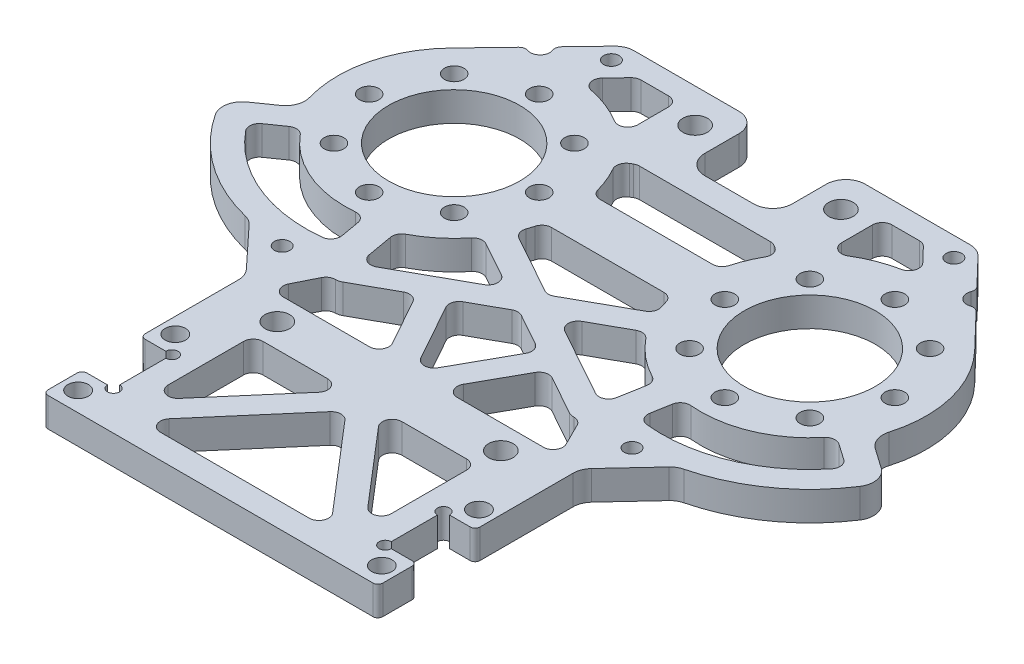
from build123d import *

# Parameters (mm, degrees)
SKETCH_1_R              = 13.5
SKETCH_1_R_2            = 2.525
SKETCH_1_R_3            = 2.01
SKETCH_1_R_4            = 2.1
SKETCH_1_R_5            = 1.6
EXTRUDE_1_DEPTH         = 6
CUT_EXTRUDE_1_DEPTH     = 111.547291087
FILLET_R2_R             = 2
FILLET_R1_R             = 1
FILLET_R4_R             = 4
CUT_EXTRUDE_73_20_DEPTH = 110.7530004


with BuildPart() as part:
    # 草图1 → 凸台-拉伸1 (new body)
    with BuildSketch(Plane(origin=(0, 0, 0), x_dir=(1, 0, 0), z_dir=(0, 1, 0))):
        with BuildLine():
            Line((-36.261062267, 35), (-9, 35))
            Line((-9, 35), (-9, 20))
            Line((-9, 20), (9, 20))
            Line((9, 20), (9, 35))
            Line((9, 35), (36.261062267, 35))
            Line((36.261062267, 35), (53.909452324, 16.624766472))
            ThreePointArc((53.909452324, 16.624766472), (60.203109588, 4.346632924), (58.696156922, -9.368022698))
            Line((58.696156922, -9.368022698), (68.25790113, -16.063228071))
            ThreePointArc((68.25790113, -16.063228071), (58.255238391, -28.130066659), (44.031297301, -34.713481825))
            Line((44.031297301, -34.713481825), (34.45, -45))
            Line((34.45, -45), (34.45, -66.75))
            Line((34.45, -66.75), (29.2, -66.75))
            ThreePointArc((29.2, -66.75), (27.066116524, -65.866116524), (27.95, -68))
            Line((27.95, -68), (27.95, -77.5))
            ThreePointArc((27.95, -77.5), (27.066116524, -79.633883476), (29.2, -78.75))
            Line((29.2, -78.75), (34.45, -78.75))
            Line((34.45, -78.75), (34.45, -86.75))
            Line((34.45, -86.75), (-34.45, -86.75))
            Line((-34.45, -86.75), (-34.45, -78.75))
            Line((-34.45, -78.75), (-29.2, -78.75))
            ThreePointArc((-29.2, -78.75), (-27.066116524, -79.633883476), (-27.95, -77.5))
            Line((-27.95, -77.5), (-27.95, -68))
            ThreePointArc((-27.95, -68), (-27.066116524, -65.866116524), (-29.2, -66.75))
            Line((-29.2, -66.75), (-34.45, -66.75))
            Line((-34.45, -66.75), (-34.45, -45))
            Line((-34.45, -45), (-44.031297301, -34.713481825))
            ThreePointArc((-44.031297301, -34.713481825), (-58.255238391, -28.130066659), (-68.25790113, -16.063228071))
            Line((-68.25790113, -16.063228071), (-58.696156922, -9.368022698))
            ThreePointArc((-58.696156922, -9.368022698), (-60.203109588, 4.346632924), (-53.909452324, 16.624766472))
            Line((-53.909452324, 16.624766472), (-36.261062267, 35))
        make_face()
        with Locations(Location((-36.6, 0, 0), (0, 0, 270))):
            Circle(SKETCH_1_R, mode=Mode.SUBTRACT)
        with Locations(Location((-15, 28, 0), (0, 0, 270))):
            Circle(SKETCH_1_R_2, mode=Mode.SUBTRACT)
        with Locations(Location((15, 28, 0), (0, 0, 270))):
            Circle(SKETCH_1_R_2, mode=Mode.SUBTRACT)
        with Locations(Location((-23, -50, 0), (0, 0, 270))):
            Circle(SKETCH_1_R_2, mode=Mode.SUBTRACT)
        with Locations(Location((23, -50, 0), (0, 0, 270))):
            Circle(SKETCH_1_R_2, mode=Mode.SUBTRACT)
        with Locations(Location((36.6, 0, 0), (0, 0, 90))):
            Circle(SKETCH_1_R, mode=Mode.SUBTRACT)
        with Locations(Location((-36.6, 17.5, 0), (0, 0, 270))):
            Circle(SKETCH_1_R_3, mode=Mode.SUBTRACT)
        with Locations(Location((-24.225631329, 12.374368671, 0), (0, 0, 270))):
            Circle(SKETCH_1_R_3, mode=Mode.SUBTRACT)
        with Locations(Location((-19.1, 0, 0), (0, 0, 270))):
            Circle(SKETCH_1_R_3, mode=Mode.SUBTRACT)
        with Locations(Location((-24.225631329, -12.374368671, 0), (0, 0, 270))):
            Circle(SKETCH_1_R_3, mode=Mode.SUBTRACT)
        with Locations(Location((-36.6, -17.5, 0), (0, 0, 270))):
            Circle(SKETCH_1_R_3, mode=Mode.SUBTRACT)
        with Locations(Location((-48.974368671, -12.374368671, 0), (0, 0, 270))):
            Circle(SKETCH_1_R_3, mode=Mode.SUBTRACT)
        with Locations(Location((-54.1, 0, 0), (0, 0, 270))):
            Circle(SKETCH_1_R_3, mode=Mode.SUBTRACT)
        with Locations(Location((-48.974368671, 12.374368671, 0), (0, 0, 270))):
            Circle(SKETCH_1_R_3, mode=Mode.SUBTRACT)
        with Locations(Location((48.974368671, 12.374368671, 0), (0, 0, 90))):
            Circle(SKETCH_1_R_3, mode=Mode.SUBTRACT)
        with Locations(Location((54.1, 0, 0), (0, 0, 90))):
            Circle(SKETCH_1_R_3, mode=Mode.SUBTRACT)
        with Locations(Location((48.974368671, -12.374368671, 0), (0, 0, 90))):
            Circle(SKETCH_1_R_3, mode=Mode.SUBTRACT)
        with Locations(Location((36.6, -17.5, 0), (0, 0, 90))):
            Circle(SKETCH_1_R_3, mode=Mode.SUBTRACT)
        with Locations(Location((24.225631329, -12.374368671, 0), (0, 0, 90))):
            Circle(SKETCH_1_R_3, mode=Mode.SUBTRACT)
        with Locations(Location((19.1, 0, 0), (0, 0, 90))):
            Circle(SKETCH_1_R_3, mode=Mode.SUBTRACT)
        with Locations(Location((24.225631329, 12.374368671, 0), (0, 0, 90))):
            Circle(SKETCH_1_R_3, mode=Mode.SUBTRACT)
        with Locations(Location((36.6, 17.5, 0), (0, 0, 90))):
            Circle(SKETCH_1_R_3, mode=Mode.SUBTRACT)
        with Locations(Location((-31.25, -82.75, 0), (0, 0, 270))):
            Circle(SKETCH_1_R_4, mode=Mode.SUBTRACT)
        with Locations(Location((-31.25, -62.75, 0), (0, 0, 270))):
            Circle(SKETCH_1_R_4, mode=Mode.SUBTRACT)
        with Locations(Location((31.25, -82.75, 0), (0, 0, 90))):
            Circle(SKETCH_1_R_4, mode=Mode.SUBTRACT)
        with Locations(Location((31.25, -62.75, 0), (0, 0, 90))):
            Circle(SKETCH_1_R_4, mode=Mode.SUBTRACT)
        with Locations(Location((-35.25, 31, 0), (0, 0, 270))):
            Circle(SKETCH_1_R_5, mode=Mode.SUBTRACT)
        with Locations(Location((35.25, 31, 0), (0, 0, 90))):
            Circle(SKETCH_1_R_5, mode=Mode.SUBTRACT)
        with Locations(Location((-36, -36, 0), (0, 0, 270))):
            Circle(SKETCH_1_R_5, mode=Mode.SUBTRACT)
        with Locations(Location((36, -36, 0), (0, 0, 90))):
            Circle(SKETCH_1_R_5, mode=Mode.SUBTRACT)
        with BuildLine():
            Line((-55.030920997, -12.905469818), (-61.584137351, -17.494081309))
            ThreePointArc((-61.584137351, -17.494081309), (-48.271844687, -28.178325742), (-31.303730581, -30.036636467))
            Line((-31.303730581, -30.036636467), (-32.692916002, -22.158174443))
            ThreePointArc((-32.692916002, -22.158174443), (-45.210377228, -20.787289482), (-55.030920997, -12.905469818))
        make_face(mode=Mode.SUBTRACT)
        with BuildLine():
            Line((55.030920997, -12.905469818), (61.584137351, -17.494081309))
            ThreePointArc((61.584137351, -17.494081309), (48.271844687, -28.178325742), (31.303730581, -30.036636467))
            Line((31.303730581, -30.036636467), (32.692916002, -22.158174443))
            ThreePointArc((32.692916002, -22.158174443), (45.210377228, -20.787289482), (55.030920997, -12.905469818))
        make_face(mode=Mode.SUBTRACT)
    extrude(amount=EXTRUDE_1_DEPTH)

    # 草图3 → 切除-拉伸1 (cut, through all)
    with BuildSketch(Plane(origin=(0, 6, 0), x_dir=(1, 0, 0), z_dir=(0, 1, 0))):
        with BuildLine():
            Line((-35.748265569, 23.984881664), (-29.490856678, 30.5))
            Line((-29.490856678, 30.5), (-21, 30.5))
            Line((-21, 30.5), (-21, 18.238420984))
            ThreePointArc((-21, 18.238420984), (-27.886771893, 22.362460866), (-35.748265569, 23.984881664))
        make_face()
        with BuildLine():
            ThreePointArc((35.748265569, 23.984881664), (27.886771893, 22.362460866), (21, 18.238420984))
            Line((21, 18.238420984), (21, 30.5))
            Line((21, 30.5), (29.490856678, 30.5))
            Line((29.490856678, 30.5), (35.748265569, 23.984881664))
        make_face()
        with BuildLine():
            Line((-13.126610811, 5), (13.126610811, 5))
            ThreePointArc((13.126610811, 5), (14.513085915, 9.389793725), (16.712198489, 13.434111472))
            Line((16.712198489, 13.434111472), (14, 15))
            Line((14, 15), (-14, 15))
            Line((-14, 15), (-16.712198489, 13.434111472))
            ThreePointArc((-16.712198489, 13.434111472), (-14.513085915, 9.389793725), (-13.126610811, 5))
        make_face()
        with BuildLine():
            Line((13.126610811, -5), (-13.126610811, -5))
            ThreePointArc((-13.126610811, -5), (-13.719828244, -7.245532444), (-14.527321777, -9.423209435))
            ThreePointArc((-14.527321777, -9.423209435), (-14.469211894, -9.452626985), (-14.411888075, -9.483548344))
            Line((-14.411888075, -9.483548344), (0, -17.501639796))
            Line((0, -17.501639796), (14.411888075, -9.483548344))
            ThreePointArc((14.411888075, -9.483548344), (14.469211894, -9.452626985), (14.527321777, -9.423209435))
            ThreePointArc((14.527321777, -9.423209435), (13.719828244, -7.245532444), (13.126610811, -5))
        make_face()
        with BuildLine():
            ThreePointArc((-16.842763472, -13.852855474), (-16.899262321, -13.820451295), (-16.95489785, -13.786586289))
            ThreePointArc((-16.95489785, -13.786586289), (-21.266831345, -18.463313327), (-26.655934481, -21.842975094))
            Line((-26.655934481, -21.842975094), (-24.97170536, -31.394713087))
            Line((-24.97170536, -31.394713087), (-13.806916689, -25.183153842))
            Line((-13.806916689, -25.183153842), (-5.142180472, -20.362505289))
            Line((-5.142180472, -20.362505289), (-16.842763472, -13.852855474))
        make_face()
        with BuildLine():
            ThreePointArc((-23.296885286, -36.184653565), (-24.456132251, -36.499368441), (-25.628351624, -36.237069529))
            Line((-25.628351624, -36.237069529), (-30, -45))
            Line((-30, -45), (-5.642628511, -45))
            Line((-5.642628511, -45), (-13.560695072, -30.767898791))
            Line((-13.560695072, -30.767898791), (-23.296885286, -36.184653565))
        make_face()
        Polygon((9.191387942, -28.337023394), (0, -23.223370782), (-9.191387942, -28.337023394), (0, -44.857819528), align=None)
        with BuildLine():
            ThreePointArc((26.655934481, -21.842975094), (21.266831345, -18.463313327), (16.95489785, -13.786586289))
            ThreePointArc((16.95489785, -13.786586289), (16.899262321, -13.820451295), (16.842763472, -13.852855474))
            Line((16.842763472, -13.852855474), (5.142180472, -20.362505289))
            Line((5.142180472, -20.362505289), (13.806916944, -25.183153984))
            Line((13.806916944, -25.183153984), (24.97170536, -31.394713087))
            Line((24.97170536, -31.394713087), (26.655934481, -21.842975094))
        make_face()
        with BuildLine():
            Line((30, -45), (25.628351624, -36.237069529))
            ThreePointArc((25.628351624, -36.237069529), (24.456132251, -36.499368441), (23.296885286, -36.184653565))
            Line((23.296885286, -36.184653565), (13.560695072, -30.767898791))
            Line((13.560695072, -30.767898791), (5.642628511, -45))
            Line((5.642628511, -45), (30, -45))
        make_face()
        Polygon((-3.29399812, -55), (-22.95, -77.910590426), (-22.95, -55), align=None)
        Polygon((0, -58.839409574), (19.65600188, -81.75), (-19.65600188, -81.75), align=None)
        Polygon((22.95, -55), (3.29399812, -55), (22.95, -77.910590426), align=None)
    extrude(amount=-CUT_EXTRUDE_1_DEPTH, mode=Mode.SUBTRACT)

    # R2 镂空圆角
    fillet_r2_edges = [part.edges().sort_by_distance(p)[0] for p in [
        (-13.126610811, 3, 5),
        (13.126610811, 3, 5),
        (26.655934481, 3, 21.842975094),
        (-26.655934481, 3, 21.842975094),
        (22.95, 3, 55),
        (22.95, 3, 77.910590426),
        (3.29399812, 3, 55),
        (19.65600188, 3, 81.75),
        (-19.65600188, 3, 81.75),
        (0, 3, 58.839409574),
        (-3.29399812, 3, 55),
        (-22.95, 3, 77.910590426),
        (-22.95, 3, 55),
        (-16.712198489, 3, -13.434111472),
        (14, 3, -15),
        (16.712198489, 3, -13.434111472),
        (13.126610811, 3, -5),
        (-13.126610811, 3, -5),
        (-14, 3, -15),
        (21, 3, -30.5),
        (29.490856678, 3, -30.5),
        (35.748265569, 3, -23.984881664),
        (21, 3, -18.238420984),
        (-5.142180472, 3, 20.362505289),
        (-24.97170536, 3, 31.394713087),
        (-16.95489785, 3, 13.786586289),
        (-14.527321777, 3, 9.423209435),
        (14.527321777, 3, 9.423209435),
        (16.95489785, 3, 13.786586289),
        (0, 3, 17.501639796),
        (24.97170536, 3, 31.394713087),
        (5.142180472, 3, 20.362505289),
        (5.642628511, 3, 45),
        (13.560695072, 3, 30.767898791),
        (25.628351624, 3, 36.237069529),
        (30, 3, 45),
        (-13.560695072, 3, 30.767898791),
        (-5.642628511, 3, 45),
        (-30, 3, 45),
        (-25.628351624, 3, 36.237069529),
        (0, 3, 23.223370782),
        (9.191387942, 3, 28.337023394),
        (0, 3, 44.857819528),
        (-9.191387942, 3, 28.337023394),
        (-21, 3, -30.5),
        (-21, 3, -18.238420984),
        (-35.748265569, 3, -23.984881664),
        (61.584137351, 3, 17.494081309),
        (31.303730581, 3, 30.036636467),
        (32.692916002, 3, 22.158174443),
        (55.030920997, 3, 12.905469818),
        (-31.303730581, 3, 30.036636467),
        (-61.584137351, 3, 17.494081309),
        (-55.030920997, 3, 12.905469818),
        (-32.692916002, 3, 22.158174443),
        (-29.490856678, 3, -30.5),
    ]]
    fillet(fillet_r2_edges, radius=FILLET_R2_R)

    # R1 插接圆角
    fillet_r1_edges = [part.edges().sort_by_distance(p)[0] for p in [
        (34.45, 3, 86.75),
        (-34.45, 3, 86.75),
        (-34.45, 3, 78.75),
        (-34.45, 3, 66.75),
        (34.45, 3, 66.75),
        (34.45, 3, 78.75),
    ]]
    fillet(fillet_r1_edges, radius=FILLET_R1_R)

    # R4 外缘圆角
    fillet_r4_edges = [part.edges().sort_by_distance(p)[0] for p in [
        (-34.45, 3, 45),
        (-44.031297301, 3, 34.713481825),
        (-68.25790113, 3, 16.063228071),
        (-58.696156922, 3, 9.368022698),
        (-36.261062267, 3, -35),
        (-9, 3, -35),
        (-9, 3, -20),
        (9, 3, -20),
        (9, 3, -35),
        (36.261062267, 3, -35),
        (58.696156922, 3, 9.368022698),
        (68.25790113, 3, 16.063228071),
        (44.031297301, 3, 34.713481825),
        (34.45, 3, 45),
    ]]
    fillet(fillet_r4_edges, radius=FILLET_R4_R)

    # 草图4 → 73.20标识 (cut, through all)
    with BuildSketch(Plane(origin=(0, 6, 0), x_dir=(1, 0, 0), z_dir=(0, 1, 0))):
        with BuildLine():
            Line((-42.714556509, 28.2807206), (-47.095567144, 23.7192794))
            ThreePointArc((-47.095567144, 23.7192794), (-46.372654237, 24.136655469), (-45.538584425, 24.102989426))
            ThreePointArc((-45.538584425, 24.102989426), (-43.462607466, 24.614602794), (-43.035149776, 26.709527254))
            ThreePointArc((-43.035149776, 26.709527254), (-43.102432535, 27.541560237), (-42.714556509, 28.2807206))
        make_face()
        with BuildLine():
            Line((42.714556509, 28.2807206), (47.095567144, 23.7192794))
            ThreePointArc((47.095567144, 23.7192794), (46.372654237, 24.136655469), (45.538584425, 24.102989426))
            ThreePointArc((45.538584425, 24.102989426), (43.462607466, 24.614602794), (43.035149776, 26.709527254))
            ThreePointArc((43.035149776, 26.709527254), (43.102432535, 27.541560237), (42.714556509, 28.2807206))
        make_face()
    extrude(amount=-CUT_EXTRUDE_73_20_DEPTH, mode=Mode.SUBTRACT)


solid = part.part
